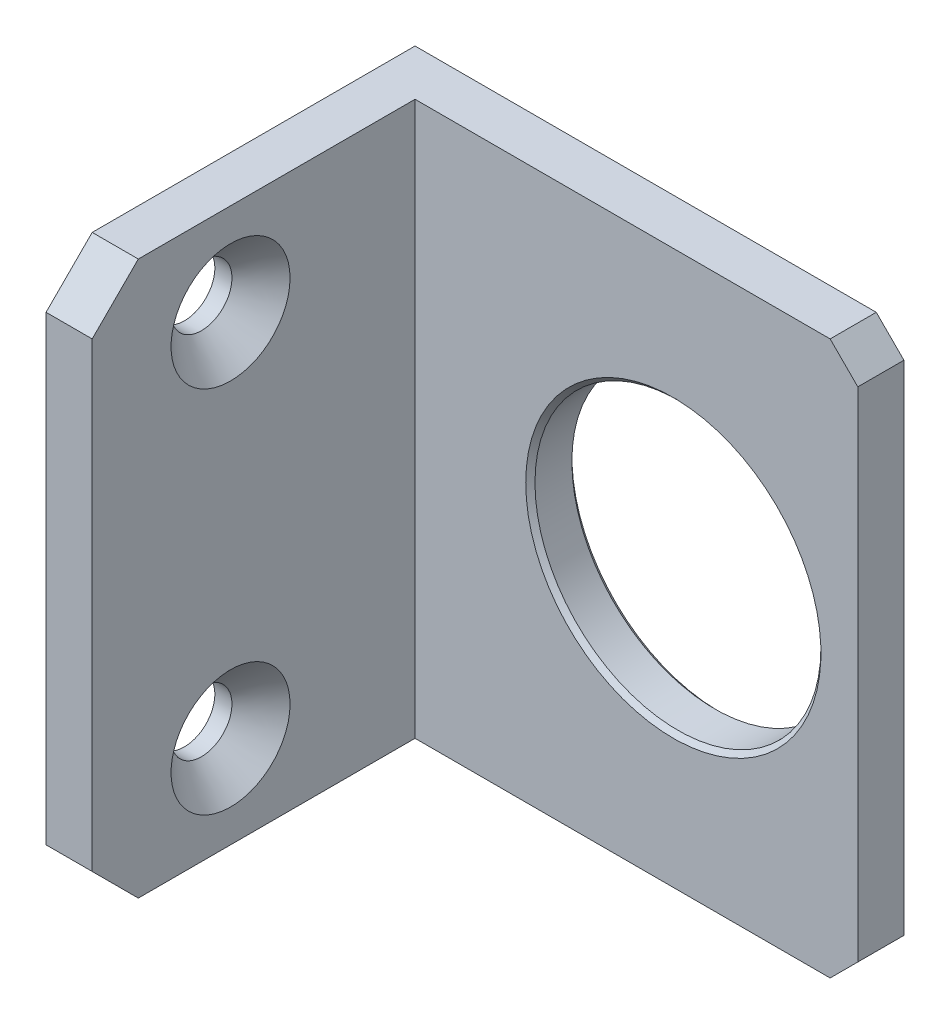
from build123d import *

# Parameters (mm, degrees)
EXTRUDE_1_DEPTH          = 60
SKETCH_2_R               = 15.5
CUT_EXTRUDE_1_DEPTH      = 90.493016487
CHAMFER_1_SIZE           = 3
CHAMFER_2_SIZE           = 5
HOLE_WIZARD_1_AT_2_COUNT = 2
HOLE_WIZARD_1_AT_2_PITCH = 40
CHAMFER_3_SIZE           = 0.5


with BuildPart() as part:
    # 草图1 → 凸台-拉伸1 (new body)
    with BuildSketch(Plane(origin=(0, 0, 0), x_dir=(1, 0, 0), z_dir=(0, 1, 0))):
        Polygon((0, 0), (0, 40), (53, 40), (53, 35), (5, 35), (5, 0), align=None)
    extrude(amount=EXTRUDE_1_DEPTH)

    # 草图2 → 切除-拉伸1 (cut, through all)
    with BuildSketch(Plane(origin=(0, 0, -40), x_dir=(-1, 0, 0), z_dir=(0, 0, -1))):
        with Locations((-33, 30)):
            Circle(SKETCH_2_R)
    extrude(amount=-CUT_EXTRUDE_1_DEPTH, mode=Mode.SUBTRACT)

    # 倒角1
    chamfer_1_edges = [part.edges().sort_by_distance(p)[0] for p in [
        (53, 60, -37.5),
        (53, 0, -37.5),
    ]]
    chamfer(chamfer_1_edges, length=CHAMFER_1_SIZE)

    # 倒角2
    chamfer_2_edges = [part.edges().sort_by_distance(p)[0] for p in [
        (2.5, 60, 0),
        (2.5, 0, 0),
    ]]
    chamfer(chamfer_2_edges, length=CHAMFER_2_SIZE)

    # 草图3 → 打孔尺寸根据十字槽沉头木螺钉的类型1 (revolve, cut)
    with BuildSketch(Plane(origin=(5, 10, -15), x_dir=(0, 0, -1), z_dir=(0, 1, 0))):
        Polygon((0, 0), (0, 5), (3.3, 5), (3.3, 3.15), (6.45, 0), align=None)
    hole_wizard_1 = revolve(axis=Axis((11.35, 10, -15), (-1, 0, 0)), mode=Mode.SUBTRACT)

    # 打孔尺寸根据十字槽沉头木螺钉的类型1 at 2: 打孔尺寸根据十字槽沉头木螺钉的类型1 ×2
    with Locations(*[(0, i * HOLE_WIZARD_1_AT_2_PITCH, 0) for i in range(1, HOLE_WIZARD_1_AT_2_COUNT)]):
        add(hole_wizard_1, mode=Mode.SUBTRACT)

    # 倒角3
    chamfer_3_edges = [part.edges().sort_by_distance(p)[0] for p in [
        (48.5, 30, -35),
        (48.5, 30, -40),
    ]]
    chamfer(chamfer_3_edges, length=CHAMFER_3_SIZE)


solid = part.part
